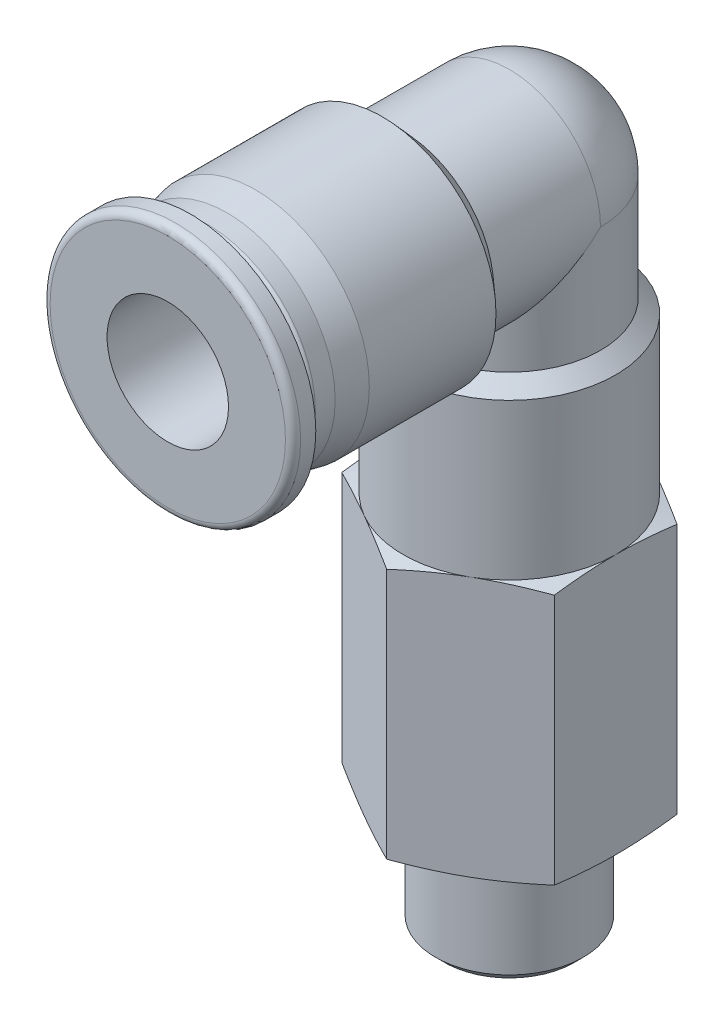
from build123d import *

# Parameters (mm, degrees)
SKETCH_3_R          = 14
CUT_EXTRUDE_1_DEPTH = 21.4
SKETCH_5_W          = 2.666666667
SKETCH_5_H          = 42.8


with BuildPart() as part:
    # 草图1 → 旋转1 (revolve)
    with BuildSketch(Plane(origin=(0, 0, 0), x_dir=(0, 0, -1), z_dir=(1, 0, 0)), mode=Mode.PRIVATE) as revolve_1_sk:
        with BuildLine():
            Line((-22.5, 0), (-22.5, 7.75))
            ThreePointArc((-22.5, 7.75), (-22.353553391, 8.103553391), (-22, 8.25))
            Line((-22, 8.25), (-21, 8.25))
            Line((-21, 8.25), (-21, 6))
            Line((-21, 6), (-20.1, 6))
            Line((-20.1, 6), (-20.1, 6.925))
            ThreePointArc((-20.1, 6.925), (-20.041421356, 7.066421356), (-19.9, 7.125))
            Line((-19.9, 7.125), (-18.6, 7.125))
            Line((-18.6, 7.125), (-16.725, 7.5))
            Line((-16.725, 7.5), (-8.381856066, 7.5))
            Line((-8.381856066, 7.5), (-7.03125, 6))
            Line((-7.03125, 6), (0, 6))
            ThreePointArc((0, 6), (4.242640687, 4.242640687), (6, 0))
            Line((6, 0), (-22.5, 0))
        make_face()
    revolve(revolve_1_sk.sketch.rotate(Axis((0, 0, -6), (0, 0, 1)), 270), axis=Axis((0, 0, -6), (0, 0, 1)))

    # 草图2 → 旋转2 (revolve)
    with BuildSketch(Plane(origin=(0, 0, 0), x_dir=(0, 0, -1), z_dir=(1, 0, 0)), mode=Mode.PRIVATE) as revolve_2_sk:
        Polygon((0, -42.8), (-4.283, -42.8), (-4.864, -42.219), (-4.864, -35.872339475), (-8.082903769, -35.00983681), (-8.082903769, -18.47016319), (-7, -18.18), (-7, -7.931654044), (-6, -7.03125), (-6, 0), (0, 0), align=None)
    revolve(revolve_2_sk.sketch.rotate(Axis((0, 0, 0), (0, -1, 0)), 180), axis=Axis((0, 0, 0), (0, -1, 0)))

    # 草图3 → 切除-拉伸1 (cut)
    with BuildSketch(Plane(origin=(0, -35.3, 0), x_dir=(1, 0, 0), z_dir=(0, 1, 0))):
        Circle(SKETCH_3_R)
        Polygon((-7, 4.041451884), (-7, -4.041451884), (0, -8.082903769), (7, -4.041451884), (7, 4.041451884), (0, 8.082903769), align=None, mode=Mode.SUBTRACT)
    extrude(amount=CUT_EXTRUDE_1_DEPTH, mode=Mode.SUBTRACT)

    # 草图4 → 切除-旋转1 (revolve, cut)
    with BuildSketch(Plane(origin=(0, 0, 0), x_dir=(0, 0, -1), z_dir=(1, 0, 0)), mode=Mode.PRIVATE) as cut_revolve_1_sk:
        with BuildLine():
            Line((-22.5, 0), (-22.5, 4))
            Line((-22.5, 4), (0, 4))
            ThreePointArc((0, 4), (2.828427125, 2.828427125), (4, 0))
            Line((4, 0), (-22.5, 0))
        make_face()
    revolve(cut_revolve_1_sk.sketch.rotate(Axis((0, 0, -4), (0, 0, 1)), 270), axis=Axis((0, 0, -4), (0, 0, 1)), mode=Mode.SUBTRACT)

    # 草图5 → 切除-旋转2 (revolve, cut)
    with BuildSketch(Plane(origin=(0, 0, 0), x_dir=(0, 0, -1), z_dir=(1, 0, 0)), mode=Mode.PRIVATE) as cut_revolve_2_sk:
        with Locations((-1.333333334, -21.4)):
            Rectangle(SKETCH_5_W, SKETCH_5_H)
    revolve(cut_revolve_2_sk.sketch.rotate(Axis((0, 0, 0), (0, -1, 0)), 180), axis=Axis((0, 0, 0), (0, -1, 0)), mode=Mode.SUBTRACT)


solid = part.part
